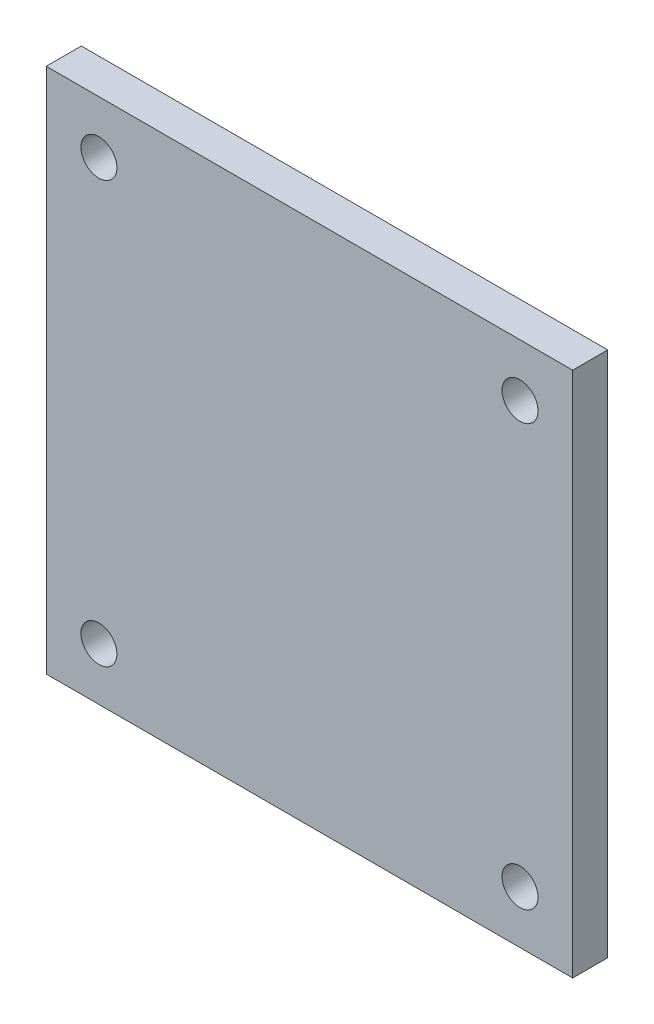
from build123d import *

# Parameters (mm, degrees)
SKETCH1_W               = 30
SKETCH1_H               = 30
BOSS_EXTRUDE1_DEPTH     = 2
SKETCH2_R               = 6
BOSS_EXTRUDE2_DEPTH     = 8
SKETCH4_R               = 0.5
CUT_EXTRUDE1_DEPTH      = 10
SKETCH6_R               = 2.5
CUT_EXTRUDE3_DEPTH      = 9
CUT_EXTRUDE4_DEPTH      = 0.1
CUT_EXTRUDE4_DEPTH_BACK = 4
SKETCH7_R               = 0.5
SKETCH8_OUTSIDE_W       = 40.718
SKETCH8_OUTSIDE_H       = 40.718
SKETCH8_OUTSIDE_W_2     = 15.543966854
SKETCH8_OUTSIDE_H_2     = 10
CUT_EXTRUDE5_DEPTH      = 8
M3_TAPPED_HOLE1_D       = 2.5
M3_TAPPED_HOLE1_DEPTH   = 3
M3_TAPPED_HOLE1_TIP     = 0.751075774
M2_5_TAPPED_HOLE1_D     = 2.05


with BuildPart() as part:
    # Sketch1 → Boss-Extrude1 (new body)
    with BuildSketch(Plane.XY):
        Rectangle(SKETCH1_W, SKETCH1_H)
    extrude(amount=BOSS_EXTRUDE1_DEPTH)

    # Sketch2 → Boss-Extrude2 (add)
    with BuildSketch(Plane(origin=(0, 0, 0), x_dir=(-1, 0, 0), z_dir=(0, 0, -1))):
        Circle(SKETCH2_R)
    extrude(amount=BOSS_EXTRUDE2_DEPTH)

    # Sketch4 → Cut-Extrude1 (cut)
    with BuildSketch(Plane.XY.offset(2)):
        with Locations((-12, 12)):
            Circle(SKETCH4_R)
        with Locations((12, 12)):
            Circle(SKETCH4_R)
        with Locations((12, -12)):
            Circle(SKETCH4_R)
        with Locations((-12, -12)):
            Circle(SKETCH4_R)
    extrude(amount=-CUT_EXTRUDE1_DEPTH, mode=Mode.SUBTRACT)

    # Sketch6 → Cut-Extrude3 (cut)
    with BuildSketch(Plane(origin=(0, 0, -8), x_dir=(-1, 0, 0), z_dir=(0, 0, -1))):
        Circle(SKETCH6_R)
    extrude(amount=-CUT_EXTRUDE3_DEPTH, mode=Mode.SUBTRACT)

    # Sketch7 → Cut-Extrude4 (cut, two sides: drawn at the far end of the back side and taken through both)
    with BuildSketch(Plane(origin=(0, 0, 0), x_dir=(1, 0, 0), z_dir=(0, 1, 0)).offset(-CUT_EXTRUDE4_DEPTH_BACK)):
        with Locations(Location((0, 5.5, 0), (0, 0, 270))):
            Circle(SKETCH7_R)
    extrude(amount=CUT_EXTRUDE4_DEPTH + CUT_EXTRUDE4_DEPTH_BACK, mode=Mode.SUBTRACT)

    # Sketch8 outside → Cut-Extrude5 (cut)
    with BuildSketch(Plane(origin=(0, 0, -8), x_dir=(-1, 0, 0), z_dir=(0, 0, -1))):
        Rectangle(SKETCH8_OUTSIDE_W, SKETCH8_OUTSIDE_H)
        Rectangle(SKETCH8_OUTSIDE_W_2, SKETCH8_OUTSIDE_H_2, mode=Mode.SUBTRACT)
    extrude(amount=-CUT_EXTRUDE5_DEPTH, mode=Mode.SUBTRACT)

    # M3 Tapped Hole1
    with Locations(Plane(origin=(0, -5, 0), x_dir=(-1, 0, 0), z_dir=(0, -1, 0))):
        with Locations((0, 5.5)):
            Hole(M3_TAPPED_HOLE1_D / 2, depth=M3_TAPPED_HOLE1_DEPTH)
            with Locations((0, 0, -(M3_TAPPED_HOLE1_DEPTH + M3_TAPPED_HOLE1_TIP / 2))):  # 118° drill point
                Cone(0, M3_TAPPED_HOLE1_D / 2, M3_TAPPED_HOLE1_TIP, mode=Mode.SUBTRACT)

    # M2.5 Tapped Hole1 (through all)
    with Locations(Plane.XY.offset(2)):
        with Locations((12, 12), (12, -12), (-12, -12), (-12, 12)):
            Hole(M2_5_TAPPED_HOLE1_D / 2)


solid = part.part
